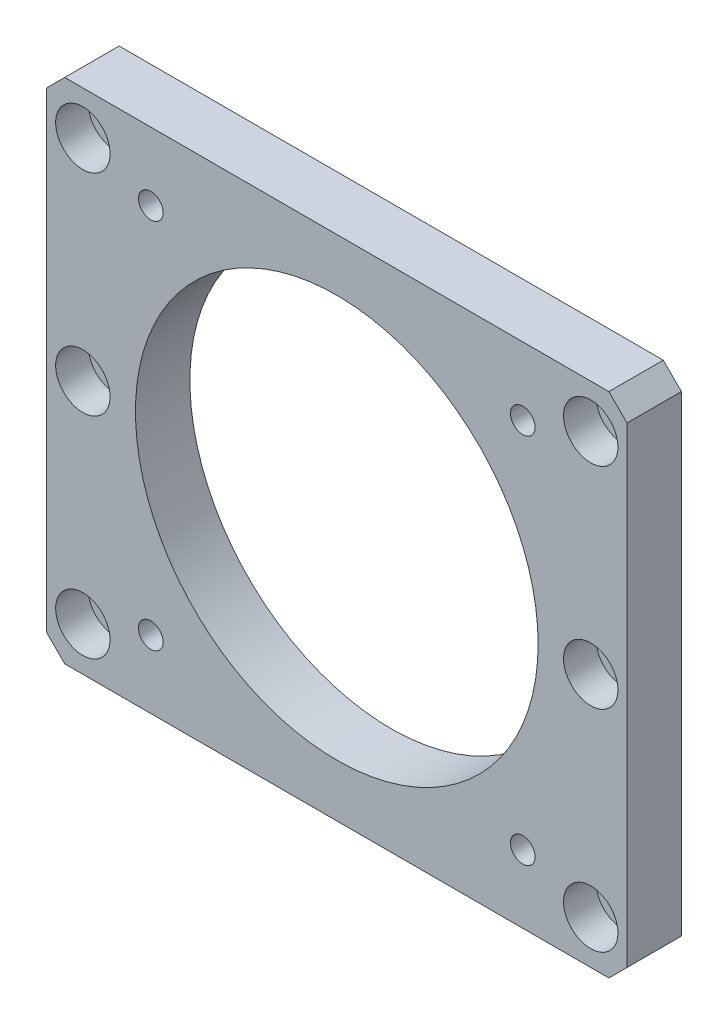
from build123d import *

# Parameters (mm, degrees)
SKETCH1_R                                            = 55.5
BOSS_EXTRUDE1_DEPTH                                  = 15
CIRPATTERN1_COUNT                                    = 4
HOLE_SIZE_PER_SOCKET_HEAD_CAP_SCREW_TYPE_D           = 9
HOLE_SIZE_PER_SOCKET_HEAD_CAP_SCREW_TYPE_CBORE_D     = 15
HOLE_SIZE_PER_SOCKET_HEAD_CAP_SCREW_TYPE_CBORE_DEPTH = 9


with BuildPart() as part:
    # Sketch1 → Boss-Extrude1 (new body)
    with BuildSketch(Plane.XY):
        Polygon((-80, 65), (-75, 70), (75, 70), (80, 65), (80, -65), (75, -70), (-75, -70), (-80, -65), align=None)
        Circle(SKETCH1_R, mode=Mode.SUBTRACT)
    extrude(amount=BOSS_EXTRUDE1_DEPTH)

    # Sketch2 → M8 Tapped Hole1 (revolve, cut)
    with BuildSketch(Plane(origin=(51.265241636, 51.265241636, 15), x_dir=(0, -1, 0), z_dir=(1, 0, 0))):
        Polygon((0, 0), (0, 21.792926105), (3.4, 19.75), (3.4, 0), align=None)
    m8_tapped_hole1 = revolve(axis=Axis((51.265241636, 51.265241636, 21.35), (0, 0, -1)), mode=Mode.SUBTRACT)

    # CirPattern1: M8 Tapped Hole1 ×4 about axis
    cirpattern1_axis = Axis((0, 0, 0), (0, 0, 1))
    for i in range(1, CIRPATTERN1_COUNT):
        add(m8_tapped_hole1.rotate(cirpattern1_axis, i * 360 / CIRPATTERN1_COUNT), mode=Mode.SUBTRACT)

    # Hole size per socket head cap screw type1 (through all)
    with Locations(Plane(origin=(37.833357844, 52.116019714, 15), x_dir=(-1, 0, 0), z_dir=(0, 0, 1))):
        with Locations((-32.166642156, -5.883980286), (-32.166642156, 52.116019714), (-32.166642156, 110.116019714)):
            hole_size_per_socket_head_cap_screw_type = CounterBoreHole(HOLE_SIZE_PER_SOCKET_HEAD_CAP_SCREW_TYPE_D / 2, HOLE_SIZE_PER_SOCKET_HEAD_CAP_SCREW_TYPE_CBORE_D / 2, HOLE_SIZE_PER_SOCKET_HEAD_CAP_SCREW_TYPE_CBORE_DEPTH)

    # Mirror1: Hole size per socket head cap screw type1 across plane
    add(hole_size_per_socket_head_cap_screw_type.mirror(Plane(origin=(0, 0, 0), x_dir=(0, 0, 1), z_dir=(1, 0, 0))), mode=Mode.SUBTRACT)


solid = part.part
